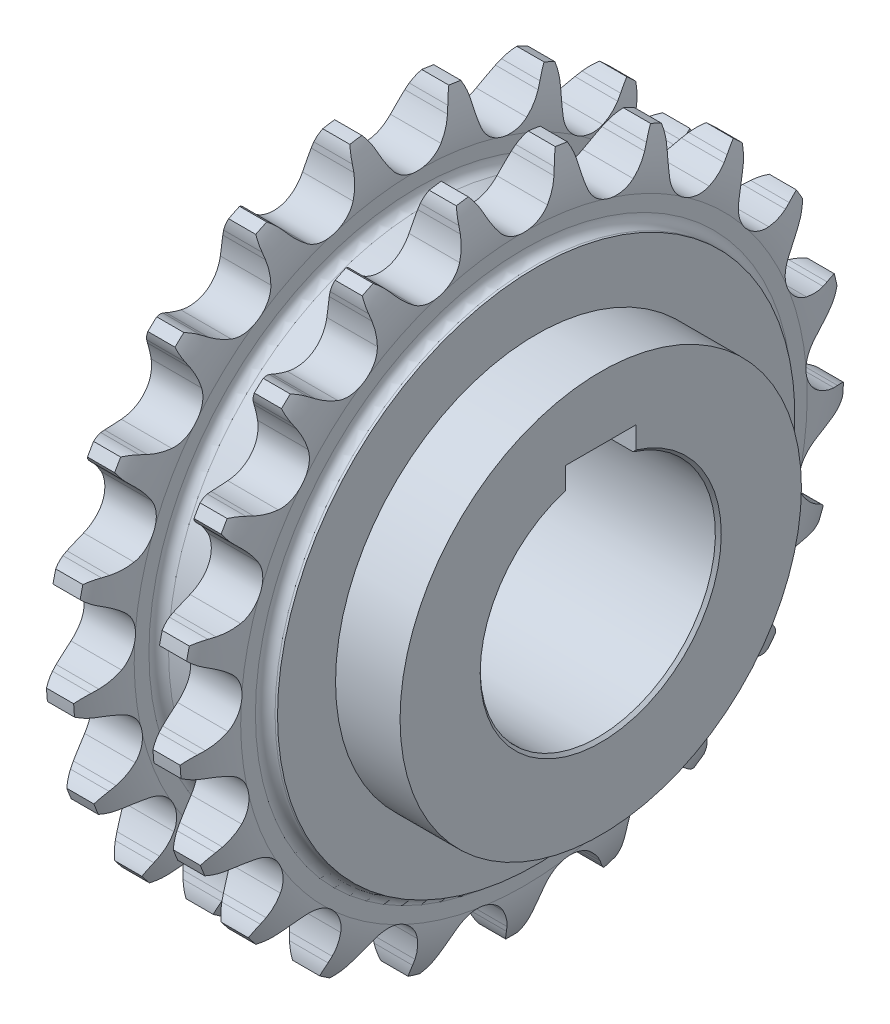
SolidWorks part; units mm, degrees
ref_plane "前视基准面" through (0, 0, 0) normal (0, 0, 1) x (1, 0, 0)
ref_plane "上视基准面" through (0, 0, 0) normal (0, 1, 0) x (1, 0, 0)
ref_plane "右视基准面" through (0, 0, 0) normal (1, 0, 0) x (0, 0, -1)
sketch "草图1" plane through (0, 0, 0) normal (0, 0, 1) x (1, 0, 0)
  line L0 (-7.9375, 0) -> (7.9375, 0) construction
  line L1 (-6.4594, 20) -> (-6.4594, 44)
  line L2 (-6.4594, 44) -> (-6.0417, 44)
  line L3 (-4.371, 45.6707) -> (-4.371, 48.1767)
  line L4 (-2.3072, 56.5) -> (2.3072, 56.5)
  line L5 (4.371, 48.1767) -> (4.371, 45.6707)
  line L6 (6.0417, 44) -> (6.4594, 44)
  line L7 (6.4594, 44) -> (6.4594, 20)
  line L8 (6.4594, 20) -> (-6.4594, 20)
  line L9 (0, 0) -> (0, 56.5) construction
  line L10 (-3.6982, 53.2567) -> (3.6982, 53.2567) construction
  line L11 (-3.6982, -53.2567) -> (3.6982, -53.2567) construction
  line L12 (7.9375, 0) -> (28.9375, 0) construction
  line L13 (-4.371, 48.1767) -> (3.7984, 48.1767) construction
  line L14 (-4.371, -48.1767) -> (3.7984, -48.1767) construction
  line L15 (28.9375, 0) -> (39.0975, 0) construction
  line L16 (39.0975, 0) -> (54.1875, 0) construction
  line L17 (54.1875, 0) -> (63.5875, 0) construction
  line L18 (63.5875, 0) -> (81.6975, 0) construction
  arc A0 (-2.3072, 56.5) -> (-4.371, 48.1767) centre (11.4966, 48.6598) ccw
  arc A1 (2.3072, 56.5) -> (4.371, 48.1767) centre (-11.4966, 48.6598) cw
  arc A2 (4.371, 45.6707) -> (6.0417, 44) centre (6.0417, 45.6707) ccw
  arc A3 (-6.0417, 44) -> (-4.371, 45.6707) centre (-6.0417, 45.6707) ccw
  point P30 (4.371, 44)
  point P33 (-4.371, 44)
  dimension "D1" = 4.1767
  dimension "rx" = 15.875
  dimension "D3" = 1.6707
  dimension "d" = 106.5134
  dimension "p" = 15.875
  dimension "z" = 21
  dimension "da" = 113
  dimension "df" = 96.3534
  dimension "dr" = 10.16
  dimension "dk" = 40
  dimension "dg" = 88
  dimension "h" = 15.09
  dimension "bf1" = 8.742
  dimension "b1" = 9.4
  dimension "ba" = 2.0638
  dimension "D2" = 2.0884
  dimension "pt" = 18.11
revolve "旋转1" add sketch "草图1" angle 360 about L0
sketch "草图2" plane through (0, 0, 0) normal (1, 0, 0) x (0, 0, -1)
  line L0 (0, 0) -> (0, 56.5) construction
  line L1 (0, 0) -> (-8.4209, 55.8689) construction
  line L2 (0, 0) -> (-16.6537, 53.9899) construction
  line L3 (4.0704, 50.0929) -> (10.2701, 45.274) construction
  line L4 (5.8527, 53.1564) -> (-6.4174, 58.2448) construction
  line L5 (0, 0) -> (8.4209, 55.8689) construction
  line L6 (5.8527, 53.1564) -> (6.2493, 54.1127)
  line L7 (-5.8527, 53.1564) -> (-6.2493, 54.1127)
  circle A0 centre (0, 0) radius 56.5 construction
  arc A1 (4.0704, 50.0929) -> (-4.0704, 50.0929) centre (0, 53.2567) cw
  arc A2 (4.0704, 50.0929) -> (5.8527, 53.1564) centre (-6.4174, 58.2448) ccw
  arc A3 (7.3999, 56.0133) -> (6.2493, 54.1127) centre (13.0605, 51.2882) ccw
  arc A4 (-4.0704, 50.0929) -> (-5.8527, 53.1564) centre (6.4174, 58.2448) cw
  arc A5 (-7.3999, 56.0133) -> (-6.2493, 54.1127) centre (-13.0605, 51.2882) cw
  arc A7 (7.3999, 56.0133) -> (-7.3999, 56.0133) centre (0, 0) ccw
  dimension "r1" = 5.1554
  dimension "r3" = 7.3736
  dimension "D1" = 17.143
  dimension "D2" = 8.571
  dimension "α/2" = 52.143
  dimension "M" = 6.4174
  dimension "T" = 4.9881
  dimension "β" = 15.333
  dimension "γ/2" = 13.952
  dimension "bc" = 1.0353
extrude "切除-拉伸1" cut sketch "草图2" against normal mid plane 12.9187
pattern_circular "阵列(圆周)1" count 21 over 360 about axis through (0, 0, 0) along (1, 0, 0) of "切除-拉伸1"
pattern_linear "阵列(线性)1" count 2 spacing 18.11 along (1, 0, 0) of bodies 103
sketch "草图7" plane through (0, 0, 0) normal (0, 0, 1) x (1, 0, 0)
  line L0 (0, 0) -> (14.4569, 0) construction
  line L1 (6.4594, 20) -> (22.8987, 20)
  line L2 (6.4594, 20) -> (6.4594, 44)
  line L3 (6.4594, 44) -> (22.8987, 44)
  line L4 (22.8987, 20) -> (22.8987, 44)
  dimension "L" = 28.9404
revolve "旋转4" add sketch "草图7" angle 360 about L0
sketch "草图3" plane through (0, 0, 0) normal (0, 0, 1) x (1, 0, 0)
  line L0 (6.4594, 20) -> (35.5406, 20)
  line L3 (35.5406, 20) -> (35.5406, 34.1318)
  line L4 (35.5406, 34.1318) -> (6.4594, 34.1318)
  line L5 (6.4594, 34.1318) -> (6.4594, 20)
  line L6 (0, 0) -> (6.4, 0) construction
  line L8 (-6.4594, 44) -> (-6.4594, -44) construction
  dimension "h" = 14.1318
  dimension "K" = 6.4
  dimension "L" = 42
revolve "旋转2" add sketch "草图3" angle 360 about L6
sketch "草图4" plane through (-6.4594, 0, 0) normal (-1, 0, 0) x (0, 0, 1)
  line L1 (-6, 19.0788) -> (6, 19.0788)
  line L2 (-6, 19.0788) -> (-6, 23.3)
  line L3 (-6, 23.3) -> (6, 23.3)
  line L4 (6, 19.0788) -> (6, 23.3)
  circle A0 centre (0, 0) radius 20 construction
  point P6 (2.7, 23.3)
  dimension "D1" = 23.3
  dimension "键槽宽度" = 12
  dimension "t1" = 3.3
extrude "切除-拉伸2" cut sketch "草图4" against normal through all
chamfer "倒角1" distance 1 angle 45 1 edges at (-6.4594, -20, 0)
chamfer "倒角3" distance 0.5 angle 45 1 edges at (35.5406, -20, 0)
